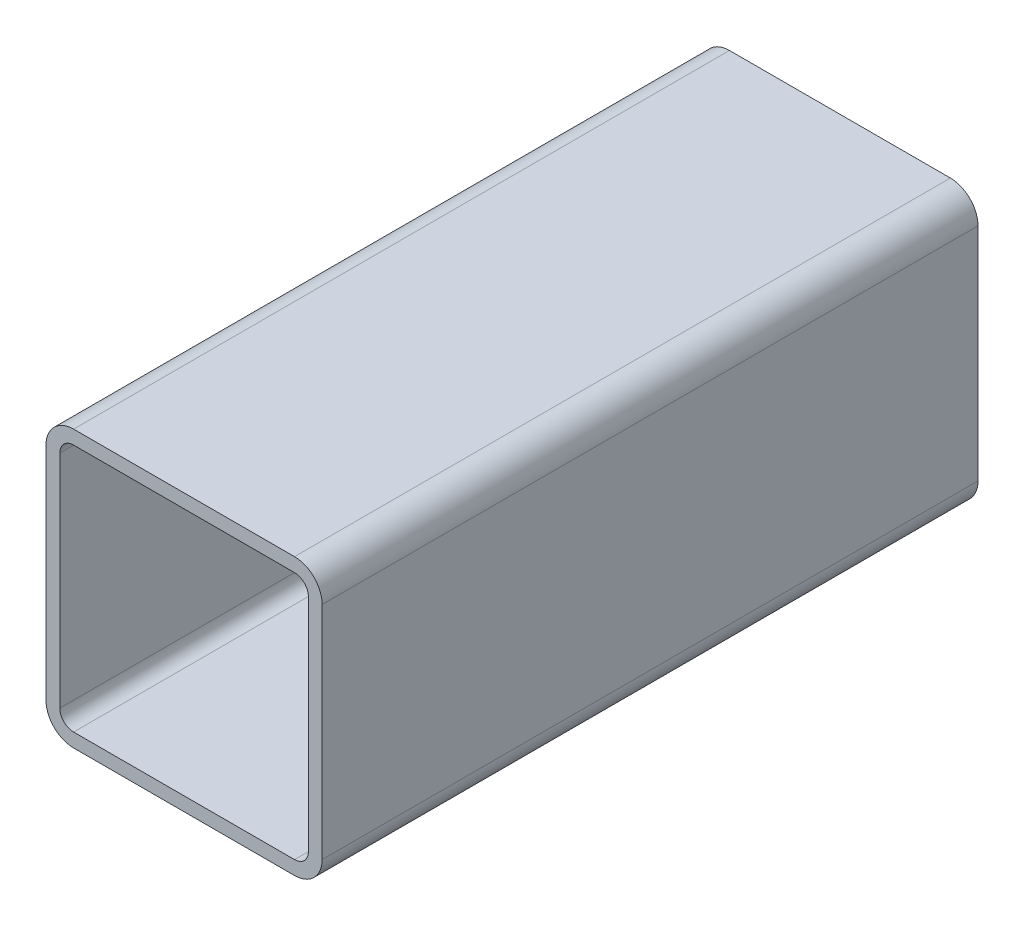
from build123d import *

# Parameters (mm, degrees)
SKETCH1_W           = 40
SKETCH1_H           = 40
SKETCH1_W_2         = 36
SKETCH1_H_2         = 36
BOSS_EXTRUDE1_DEPTH = 95
FILLET1_R           = 2
FILLET2_R           = 4


with BuildPart() as part:
    # Sketch1 → Boss-Extrude1 (new body)
    with BuildSketch(Plane.XY):
        Rectangle(SKETCH1_W, SKETCH1_H)
        Rectangle(SKETCH1_W_2, SKETCH1_H_2, mode=Mode.SUBTRACT)
    extrude(amount=BOSS_EXTRUDE1_DEPTH)

    # Fillet1
    fillet1_edges = [part.edges().sort_by_distance(p)[0] for p in [
        (18, -18, 47.5),
        (18, 18, 47.5),
        (-18, 18, 47.5),
        (-18, -18, 47.5),
    ]]
    fillet(fillet1_edges, radius=FILLET1_R)

    # Fillet2
    fillet2_edges = [part.edges().sort_by_distance(p)[0] for p in [
        (20, -20, 47.5),
        (-20, -20, 47.5),
        (-20, 20, 47.5),
        (20, 20, 47.5),
    ]]
    fillet(fillet2_edges, radius=FILLET2_R)


solid = part.part
